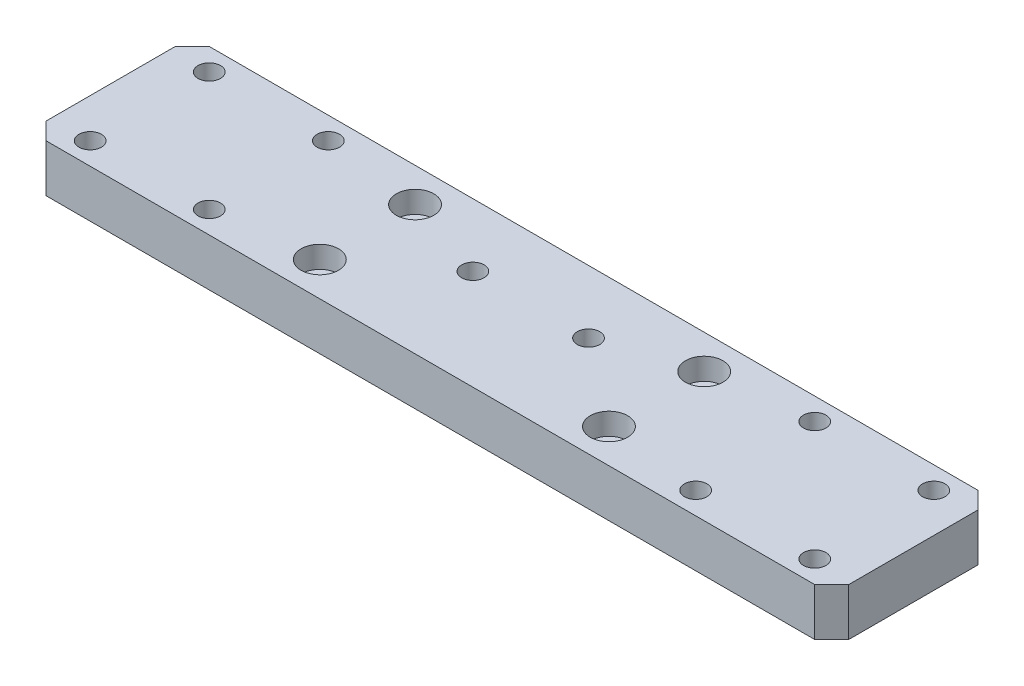
SolidWorks part; units mm, degrees
material "6061-T6"
ref_plane "前视基准面" through (0, 0, 0) normal (0, 0, 1) x (1, 0, 0)
ref_plane "上视基准面" through (0, 0, 0) normal (0, 1, 0) x (1, 0, 0)
ref_plane "右视基准面" through (0, 0, 0) normal (1, 0, 0) x (0, 0, -1)
sketch "草图2" plane through (0, 0, 0) normal (0, 0, 1) x (1, 0, 0)
  line L9 (0, 0) -> (236, 0)
  line L10 (0, 0) -> (0, -14)
  line L11 (0, -14) -> (236, -14)
  line L12 (236, 0) -> (236, -14)
  dimension "D1" = 14
  dimension "D2" = 236
extrude "凸台-拉伸1" add sketch "草图2" along normal blind 48
hole_wizard "M6 六角凹头螺钉的柱形沉头孔1" positions "草图3" profile "草图4" counterbore size "M6" standard "ISO"
sketch "草图3" plane through (0, -14, 0) normal (0, -1, 0) x (-1, 0, 0)
  line L0 (-118, -48) -> (-118, -74.0987) construction
  line L1 (0, -48) -> (-236, -48) construction
  line L3 (-224.5, -41.5) -> (-189.5, -41.5) construction
  line L4 (-189.5, -41.5) -> (-189.5, -6.5) construction
  line L5 (-189.5, -6.5) -> (-224.5, -6.5) construction
  line L6 (-224.5, -6.5) -> (-224.5, -41.5) construction
  line L8 (-236, -48) -> (-236, 0) construction
  line L9 (-224.5, -24) -> (-236, -24) construction
  point P0 (-224.5, -6.5)
  point P2 (-189.5, -6.5)
  point P4 (-189.5, -41.5)
  point P6 (-224.5, -41.5)
  point P14 (-11.5, -41.5)
  point P15 (-46.5, -41.5)
  point P16 (-46.5, -6.5)
  point P17 (-11.5, -6.5)
  dimension "D1" = 35
  dimension "D2" = 35
  dimension "D3" = 11.5
sketch "草图4" plane through (224.5, -14, 6.5) normal (1, 0, 0) x (0, 0, -1)
  line L0 (0, 0) -> (0, 15.9828)
  line L1 (0, 15.9828) -> (3.3, 14)
  line L2 (3.3, 14) -> (3.3, 6.4)
  line L3 (3.3, 6.4) -> (5.5, 6.4)
  line L4 (5.5, 6.4) -> (5.5, 0)
  line L5 (5.5, 0) -> (0, 0)
  line L10 (0, 15.9828) -> (-3.3, 14) construction
  line L11 (0, -6.35) -> (0, 107.95) construction
  dimension "孔直径" = 6.6
  dimension "孔深度" = 14
  dimension "柱形沉头孔直径" = 11
  dimension "柱形沉头孔深度" = 6.4
  dimension "导头角度" = 118
chamfer "倒角1" distance 5 angle 45 4 edges at (0, -7, 48) (0, -7, 0) (236, -7, 0) (236, -7, 48)
hole_wizard "M6 六角凹头螺钉的柱形沉头孔2" positions "草图5" profile "草图6" counterbore size "M6" standard "ISO"
sketch "草图5" plane through (0, 0, 0) normal (0, 1, 0) x (1, 0, 0)
  line L0 (75.5, -38) -> (75.5, -10) construction
  line L1 (75.5, -10) -> (160.5, -10) construction
  line L2 (160.5, -10) -> (160.5, -38) construction
  line L3 (160.5, -38) -> (75.5, -38) construction
  line L5 (160.5, -24) -> (236, -24) construction
  line L6 (236, -43) -> (236, -5) construction
  line L8 (118, -38) -> (118, -48) construction
  line L9 (231, -48) -> (5, -48) construction
  point P0 (75.5, -10)
  point P2 (160.5, -10)
  point P4 (75.5, -38)
  point P6 (160.5, -38)
  dimension "D1" = 85
  dimension "D2" = 28
sketch "草图6" plane through (75.5, 0, 10) normal (1, 0, 0) x (0, 0, 1)
  line L0 (0, 0) -> (0, 15.9828)
  line L1 (0, 15.9828) -> (3.3, 14)
  line L2 (3.3, 14) -> (3.3, 6.4)
  line L3 (3.3, 6.4) -> (5.5, 6.4)
  line L4 (5.5, 6.4) -> (5.5, 0)
  line L5 (5.5, 0) -> (0, 0)
  line L10 (0, 15.9828) -> (-3.3, 14) construction
  line L11 (0, -6.35) -> (0, 107.95) construction
  dimension "孔直径" = 6.6
  dimension "孔深度" = 14
  dimension "柱形沉头孔直径" = 11
  dimension "柱形沉头孔深度" = 6.4
  dimension "导头角度" = 118
hole_wizard "M6 间隙孔1" positions "草图7" profile "草图8" hole size "M6" standard "ISO" end condition through all
sketch "草图7" plane through (0, 0, 0) normal (0, 1, 0) x (1, 0, 0)
  line L0 (101, -18.5) -> (135, -18.5) construction
  line L2 (118, -18.5) -> (118, 0) construction
  line L3 (231, 0) -> (5, 0) construction
  point P0 (101, -18.5)
  point P2 (135, -18.5)
  dimension "D1" = 18.5
  dimension "D2" = 34
sketch "草图8" plane through (101, 0, 18.5) normal (1, 0, 0) x (0, 0, 1)
  line L0 (0, 0) -> (0, 14)
  line L1 (0, 14) -> (3.3, 14)
  line L2 (3.3, 14) -> (3.3, 0)
  line L5 (3.3, 0) -> (0, 0)
  line L11 (0, -6.35) -> (0, 107.95) construction
  dimension "通孔孔直径" = 6.6
  dimension "通孔孔深度" = 14
